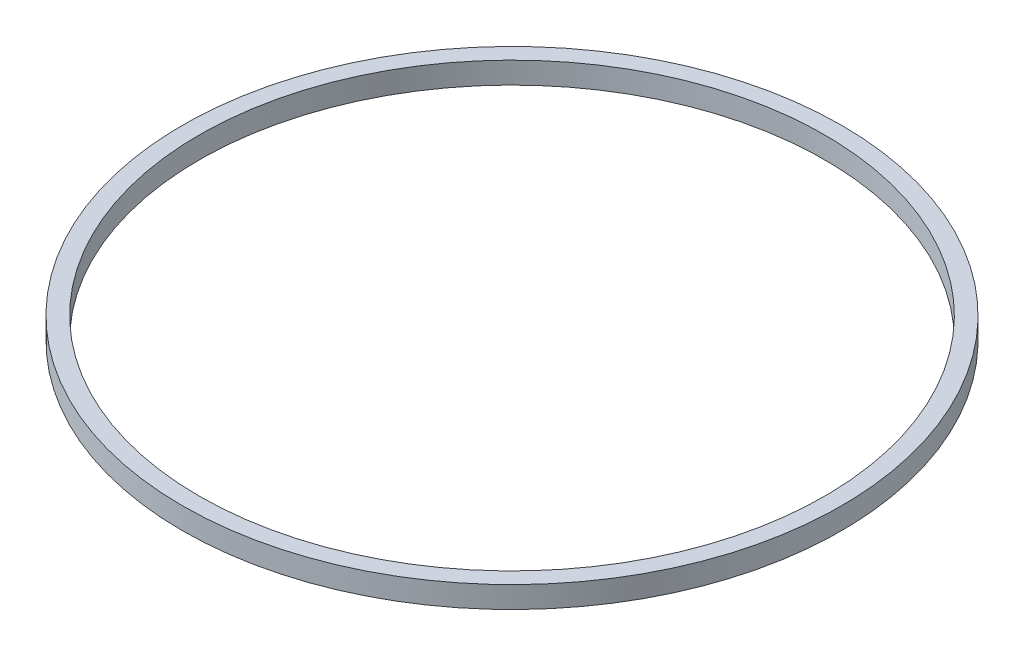
SolidWorks part; units mm, degrees
material "轻木"
ref_plane "前视基准面" through (0, 0, 0) normal (0, 0, 1) x (1, 0, 0)
ref_plane "上视基准面" through (0, 0, 0) normal (0, 1, 0) x (1, 0, 0)
ref_plane "右视基准面" through (0, 0, 0) normal (1, 0, 0) x (0, 0, -1)
other "Configuration Table"
sketch "草图1" plane through (0, 0, 0) normal (0, 1, 0) x (1, 0, 0)
  circle A0 centre (0, 0) radius 305
  circle A1 centre (0, 0) radius 289.5
  dimension "D1" = 610
  dimension "D2" = 579
extrude "凸台-拉伸1" add sketch "草图1" along normal blind 20
